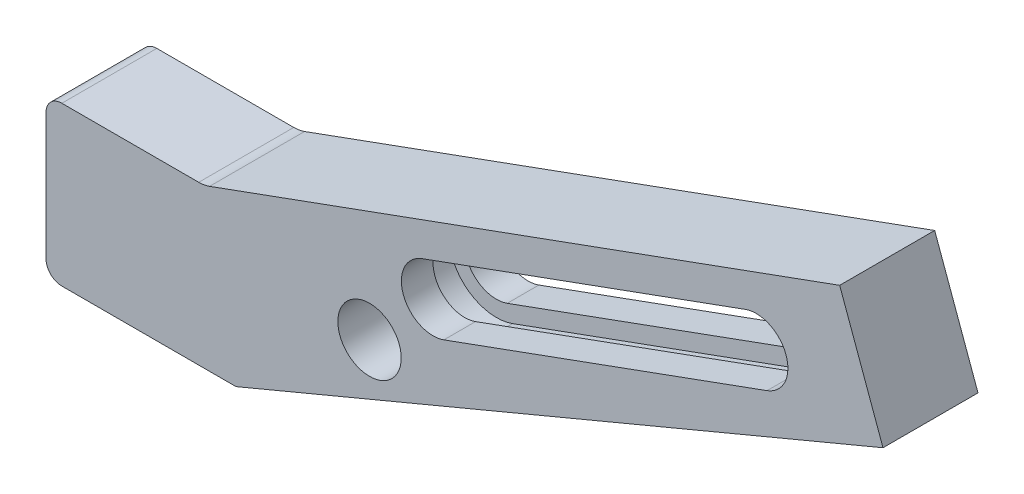
from build123d import *

# Parameters (mm, degrees)
BOSS_EXTRUDE1_DEPTH = 15
FILLET1_R           = 10
FILLET2_R           = 5
SKETCH2_R           = 5
CUT_EXTRUDE1_DEPTH  = 10
SKETCH3_R           = 5
CUT_EXTRUDE2_DEPTH  = 10
SKETCH5_R           = 10
BOSS_EXTRUDE3_DEPTH = 10
SKETCH6_R           = 7.5
BOSS_EXTRUDE4_DEPTH = 5
SKETCH7_R           = 10
BOSS_EXTRUDE5_DEPTH = 2
SKETCH8_R           = 10
CUT_EXTRUDE3_DEPTH  = 80
CUT_EXTRUDE4_DEPTH  = 5
SKETCH10_W          = 33.070840011
SKETCH10_H          = 51.47652372
CUT_EXTRUDE5_DEPTH  = 50


with BuildPart() as part:
    # Sketch1 → Boss-Extrude1 (new, symmetric)
    with BuildSketch(Plane.XY):
        Polygon((0, 0), (0, 50), (50, 50), (250.63503339, 123.025180105), (264.315839123, 85.437475274), (60, 0), align=None)
        with BuildLine():
            Line((118.808982902, 64.402643902), (220.866512245, 101.548546765))
            ThreePointArc((220.866512245, 101.548546765), (233.683639886, 95.571821991), (227.706915111, 82.75469435))
            Line((227.706915111, 82.75469435), (125.649385769, 45.608791486))
            ThreePointArc((125.649385769, 45.608791486), (112.832258128, 51.585516261), (118.808982902, 64.402643902))
        make_face(mode=Mode.SUBTRACT)
    extrude(amount=BOSS_EXTRUDE1_DEPTH, both=True)

    # Fillet1
    fillet1_edges = [part.edges().sort_by_distance(p)[0] for p in [
        (50, 50, 0),
    ]]
    fillet(fillet1_edges, radius=FILLET1_R)

    # Fillet2
    fillet2_edges = [part.edges().sort_by_distance(p)[0] for p in [
        (0, 0, 0),
        (0, 50, 0),
    ]]
    fillet(fillet2_edges, radius=FILLET2_R)

    # Sketch2 → Cut-Extrude1 (cut)
    with BuildSketch(Plane(origin=(1.166172543, 1.605098805, 0), x_dir=(0, 0, -1), z_dir=(-0.587785252292477, -0.8090169943749446, 0))):
        with Locations(Location((0, 0, 0), (0, 0, 90))):
            Circle(SKETCH2_R)
    extrude(amount=-CUT_EXTRUDE1_DEPTH, mode=Mode.SUBTRACT)

    # Sketch3 → Cut-Extrude2 (cut)
    with BuildSketch(Plane.ZY):
        with Locations((0, 40)):
            Circle(SKETCH3_R)
    extrude(amount=-CUT_EXTRUDE2_DEPTH, mode=Mode.SUBTRACT)

    # Sketch5 → Boss-Extrude3 (add)
    with BuildSketch(Plane(origin=(0, 0, -15), x_dir=(-1, 0, 0), z_dir=(0, 0, -1))):
        with Locations((-15, 25.111581997)):
            Circle(SKETCH5_R)
    extrude(amount=BOSS_EXTRUDE3_DEPTH)

    # Sketch6 → Boss-Extrude4 (add)
    with BuildSketch(Plane(origin=(0, 0, -25), x_dir=(-1, 0, 0), z_dir=(0, 0, -1))):
        with Locations((-15, 25.111581997)):
            Circle(SKETCH6_R)
    extrude(amount=BOSS_EXTRUDE4_DEPTH)

    # Sketch7 → Boss-Extrude5 (add)
    with BuildSketch(Plane(origin=(0, 0, -30), x_dir=(-1, 0, 0), z_dir=(0, 0, -1))):
        with Locations((-15, 25.111581997)):
            Circle(SKETCH7_R)
    extrude(amount=BOSS_EXTRUDE5_DEPTH)

    # Sketch8 → Cut-Extrude3 (cut)
    with BuildSketch(Plane.XY.offset(15)):
        with Locations((102.166886521, 33.891313111)):
            Circle(SKETCH8_R)
    extrude(amount=-CUT_EXTRUDE3_DEPTH, mode=Mode.SUBTRACT)

    # Sketch9 → Cut-Extrude4 (cut, symmetric)
    with BuildSketch(Plane.XY):
        with BuildLine():
            Line((127.359486485, 40.910328382), (229.417015828, 78.056231246))
            ThreePointArc((229.417015828, 78.056231246), (238.38210299, 97.281922707), (219.156411528, 106.247009869))
            Line((219.156411528, 106.247009869), (117.098882186, 69.101107006))
            ThreePointArc((117.098882186, 69.101107006), (108.133795024, 49.875415544), (127.359486485, 40.910328382))
        make_face()
        with BuildLine():
            Line((220.866512245, 101.548546765), (118.808982902, 64.402643902))
            ThreePointArc((118.808982902, 64.402643902), (112.832258128, 51.585516261), (125.649385769, 45.608791486))
            Line((125.649385769, 45.608791486), (227.706915111, 82.75469435))
            ThreePointArc((227.706915111, 82.75469435), (233.683639886, 95.571821991), (220.866512245, 101.548546765))
        make_face(mode=Mode.SUBTRACT)
    extrude(amount=CUT_EXTRUDE4_DEPTH, both=True, mode=Mode.SUBTRACT)

    # Sketch10 → Cut-Extrude5 (cut)
    with BuildSketch(Plane.ZY):
        with Locations((-31.535420006, 25.73826186)):
            Rectangle(SKETCH10_W, SKETCH10_H)
    extrude(amount=-CUT_EXTRUDE5_DEPTH, mode=Mode.SUBTRACT)


solid = part.part
